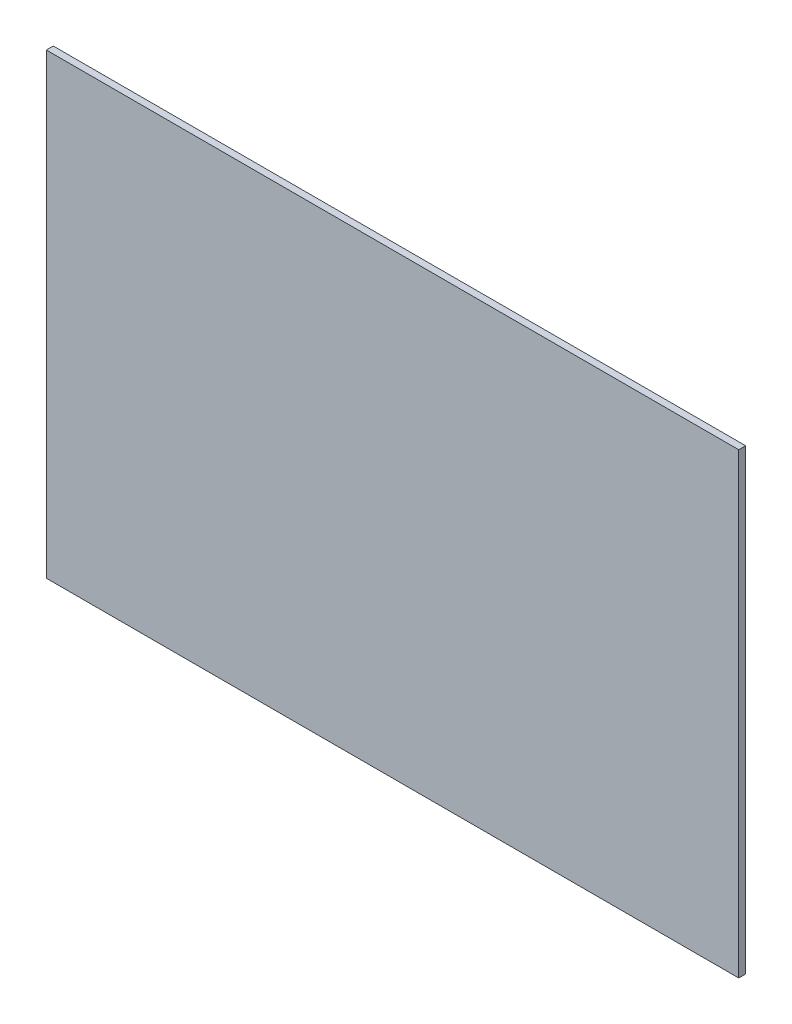
SolidWorks part; units mm, degrees
ref_plane "前视基准面" through (0, 0, 0) normal (0, 0, 1) x (1, 0, 0)
ref_plane "上视基准面" through (0, 0, 0) normal (0, 1, 0) x (1, 0, 0)
ref_plane "右视基准面" through (0, 0, 0) normal (1, 0, 0) x (0, 0, -1)
sketch "草图1" plane through (0, 0, 0) normal (0, 0, 1) x (1, 0, 0)
  line L1 (-775, 825) -> (625, 825)
  line L2 (-775, 825) -> (-775, -100)
  line L3 (-775, -100) -> (625, -100)
  line L4 (625, 825) -> (625, -100)
  point P6 (0, 0)
  point P7 (0, 0)
  dimension "D1" = 925
  dimension "D2" = 1400
extrude "凸台-拉伸1" add sketch "草图1" along normal blind 14
